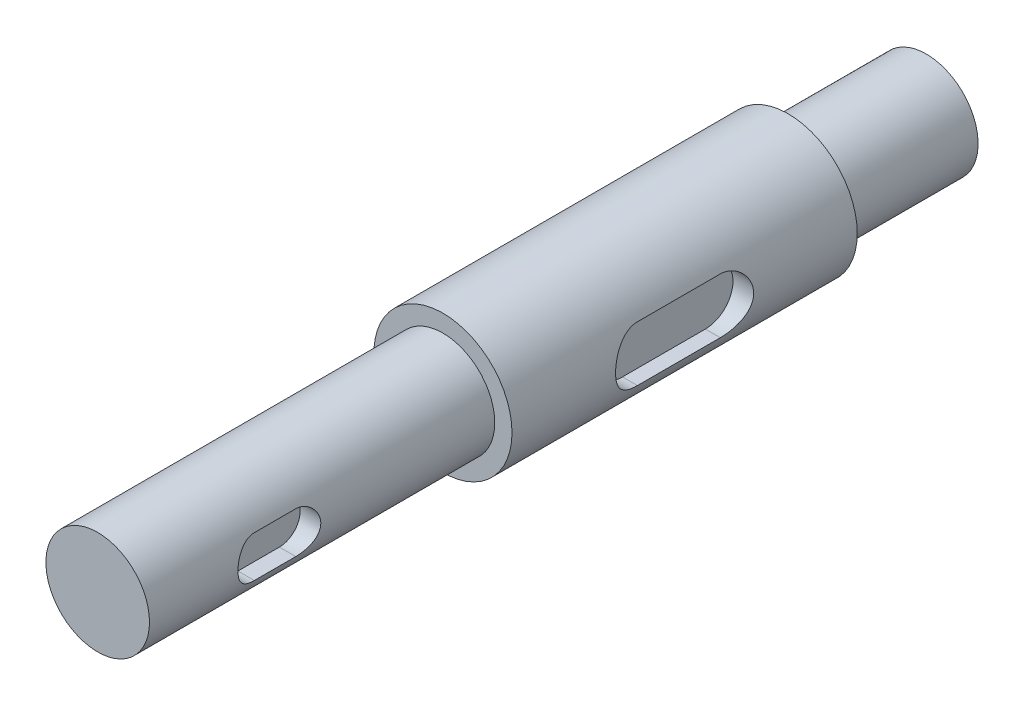
from build123d import *

# Parameters (mm, degrees)
SKETCH_1_R          = 10
EXTRUDE_1_DEPTH     = 60
SKETCH_3_R          = 7.5
EXTRUDE_3_DEPTH     = 40
CUT_EXTRUDE_START   = 10
CUT_EXTRUDE_1_DEPTH = 3
CUT_EXTRUDE_START_2 = -10
SKETCH_10_R         = 10
SKETCH_10_R_2       = 7.5
CUT_EXTRUDE_3_DEPTH = 10
CUT_EXTRUDE_START_3 = 7.5
CUT_EXTRUDE_4_DEPTH = 3
EXTRUDE_START       = 20
SKETCH_14_R         = 7.5
EXTRUDE_4_DEPTH     = 20


with BuildPart() as part:
    # 草图1 → 凸台-拉伸1 (new body)
    with BuildSketch(Plane.XY):
        with Locations(Location((0, 0, 0), (0, 0, 180))):
            Circle(SKETCH_1_R)
    extrude(amount=EXTRUDE_1_DEPTH)

    # 草图3 → 凸台-拉伸3 (add)
    with BuildSketch(Plane.XY.offset(60)):
        Circle(SKETCH_3_R)
    extrude(amount=EXTRUDE_3_DEPTH)

    # 草图4 → 切除-拉伸1 (cut)
    with BuildSketch(Plane(origin=(0, 0, 0), x_dir=(0, 0, -1), z_dir=(1, 0, 0)).offset(CUT_EXTRUDE_START)):
        with BuildLine():
            Line((-31, 4), (-19, 4))
            ThreePointArc((-19, 4), (-15, 0), (-19, -4))
            Line((-19, -4), (-31, -4))
            ThreePointArc((-31, -4), (-35, 0), (-31, 4))
        make_face()
    extrude(amount=-CUT_EXTRUDE_1_DEPTH, mode=Mode.SUBTRACT)

    # 草图10 → 切除-拉伸3 (cut)
    with BuildSketch(Plane.XY.offset(60).offset(CUT_EXTRUDE_START_2)):
        Circle(SKETCH_10_R)
        Circle(SKETCH_10_R_2, mode=Mode.SUBTRACT)
    extrude(amount=CUT_EXTRUDE_3_DEPTH, mode=Mode.SUBTRACT)

    # 草图12 → 切除-拉伸4 (cut)
    with BuildSketch(Plane(origin=(0, 0, 0), x_dir=(0, 0, -1), z_dir=(1, 0, 0)).offset(CUT_EXTRUDE_START_3)):
        with BuildLine():
            Line((-84.188029656, 3), (-78.188029656, 3))
            ThreePointArc((-78.188029656, 3), (-75.188029656, 0), (-78.188029656, -3))
            Line((-78.188029656, -3), (-84.188029656, -3))
            ThreePointArc((-84.188029656, -3), (-87.188029656, 0), (-84.188029656, 3))
        make_face()
    extrude(amount=-CUT_EXTRUDE_4_DEPTH, mode=Mode.SUBTRACT)

    # 草图14 → 凸台-拉伸4 (add)
    with BuildSketch(Plane(origin=(0, 0, 0), x_dir=(-1, 0, 0), z_dir=(0, 0, -1)).offset(EXTRUDE_START)):
        with Locations(Location((0, 0, 0), (0, 0, 180))):
            Circle(SKETCH_14_R)
    extrude(amount=-EXTRUDE_4_DEPTH)


solid = part.part
